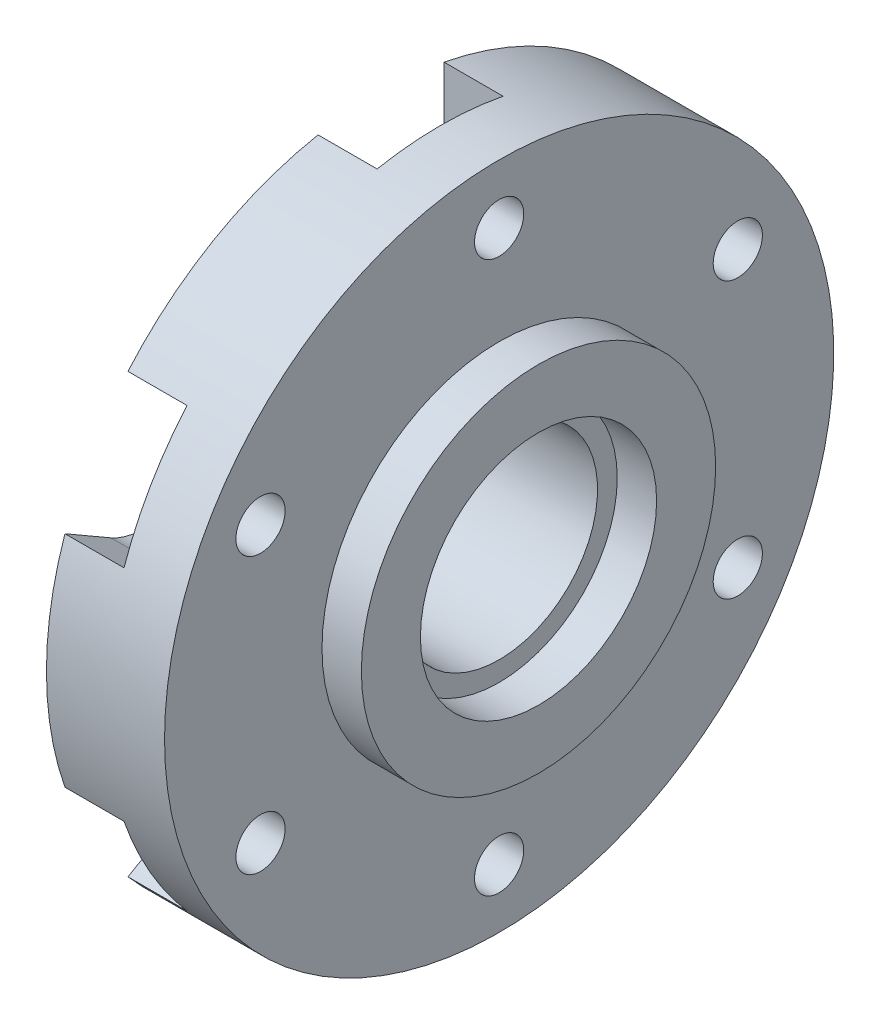
SolidWorks part; units mm, degrees
material "普通碳钢"
ref_plane "前视基准面" through (0, 0, 0) normal (0, 0, 1) x (1, 0, 0)
ref_plane "上视基准面" through (0, 0, 0) normal (0, 1, 0) x (1, 0, 0)
ref_plane "右视基准面" through (0, 0, 0) normal (1, 0, 0) x (0, 0, -1)
sketch "草图1" plane through (0, 0, 0) normal (0, 0, 1) x (1, 0, 0)
  line L0 (0, 0) -> (0, 290.7532) construction
  line L1 (0, 0) -> (356.4696, 0) construction
  line L2 (0, 0) -> (0, 85)
  line L3 (0, 85) -> (30, 85)
  line L4 (30, 85) -> (30, 45)
  line L5 (30, 45) -> (40, 45)
  line L6 (40, 45) -> (40, 30)
  line L7 (40, 30) -> (30, 30)
  line L8 (30, 30) -> (30, 0)
  line L9 (30, 0) -> (0, 0)
  dimension "D1" = 170
  dimension "D2" = 90
  dimension "D3" = 15
  dimension "D4" = 30
  dimension "D5" = 10
revolve "旋转1" add sketch "草图1" angle 360 about L1
sketch "草图2" plane through (0, 0, 0) normal (-1, 0, 0) x (0, 0, 1)
  line L0 (0, 0) -> (0, 70) construction
  circle A0 centre (0, 70) radius 6.25
  dimension "D2" = 12.5
  dimension "D1" = 70
extrude "切除-拉伸1" cut sketch "草图2" against normal through all
pattern_circular "阵列(圆周)1" count 6 over 360 about axis through (0, 0, 0) along (1, 0, 0) of "切除-拉伸1"
sketch "草图3" plane through (0, 0, 0) normal (-1, 0, 0) x (0, 0, 1)
  circle A0 centre (0, 0) radius 25
  dimension "D1" = 50
extrude "切除-拉伸2" cut sketch "草图3" against normal through all
sketch "草图6" plane through (0, 0, 0) normal (-1, 0, 0) x (0, 0, 1)
  line L0 (0, 0) -> (0, 106.2432) construction
  line L1 (-16, 70) -> (-16, 83.4805)
  line L2 (16, 70) -> (16, 83.4805)
  circle A0 centre (0, 0) radius 85 construction
  arc A1 (16, 83.4805) -> (-16, 83.4805) centre (0, 0) ccw
  arc A2 (-16, 70) -> (16, 70) centre (0, 70) ccw
  dimension "D1" = 32
extrude "切除-拉伸3" cut sketch "草图6" against normal blind 15
pattern_circular "阵列(圆周)2" count 6 over 360 about axis through (0, 0, 0) along (1, 0, 0) of "切除-拉伸3"
sketch "草图7" plane through (0, 0, 0) normal (-1, 0, 0) x (0, 0, 1)
  line L0 (0, 0) -> (0, 97.7609) construction
  line L1 (0, 0) -> (35, 60.6218) construction
  dimension "D1" = 30
  dimension "D2" = 70
hole_wizard "M12 螺纹孔1" positions "3D草图2" profile "草图8" tap size "M12" standard "GB"
sketch3d "3D草图2"
  point P0 (0, 60.6218, 35)
sketch "草图8" plane through (0, 60.6218, 35) normal (0, 1, 0) x (0, 0, 1)
  line L0 (0, 0) -> (0, 21.0644)
  line L1 (0, 21.0644) -> (5.1, 18)
  line L2 (5.1, 18) -> (5.1, 0)
  line L5 (5.1, 0) -> (0, 0)
  line L10 (0, 21.0644) -> (-5.1, 18) construction
  line L11 (0, -6.35) -> (0, 107.95) construction
  dimension "螺纹孔钻头直径" = 10.2
  dimension "螺纹孔钻头深度" = 18
  dimension "导头角度" = 118
cosmetic thread "孔螺蚊线1" parameters "D1"=15, "D2"=12
pattern_circular "阵列(圆周)3" count 6 over 360 about axis through (0, 0, 0) along (1, 0, 0) of "M12 螺纹孔1"
